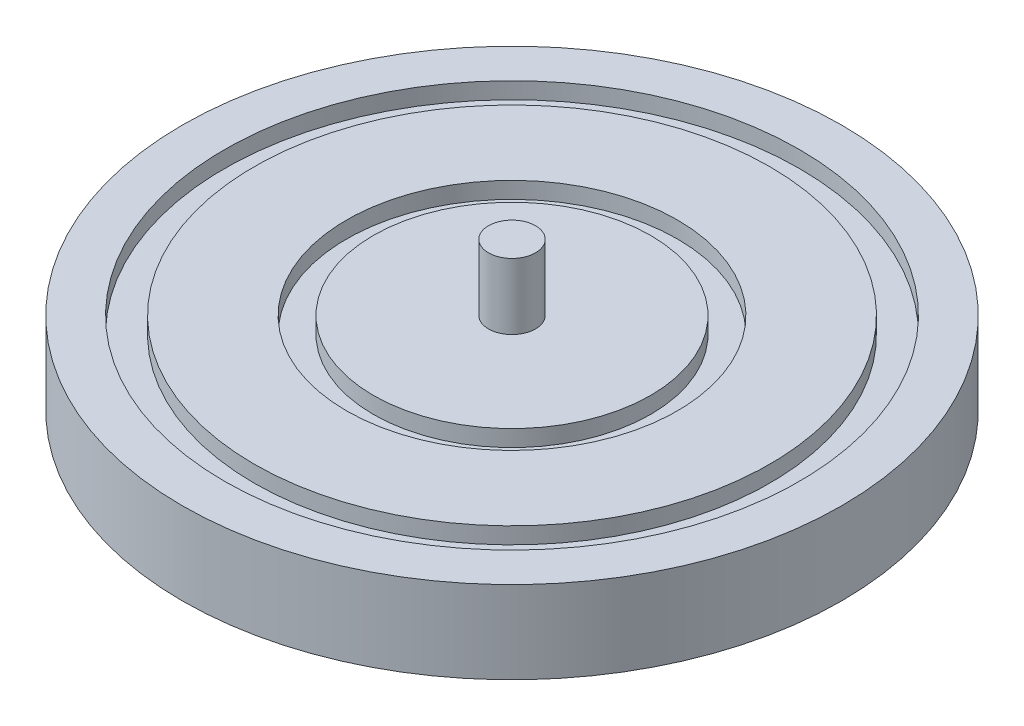
from build123d import *

# Parameters (mm, degrees)
SKETCH_1_R          = 20
EXTRUDE_1_DEPTH     = 5
SKETCH_2_R          = 5
EXTRUDE_2_DEPTH     = 6
SKETCH_3_R          = 11.669468733
SKETCH_3_R_2        = 9.545408708
CUT_EXTRUDE_1_DEPTH = 1
SKETCH_4_R          = 1.425
EXTRUDE_3_DEPTH     = 4
SKETCH_5_R          = 17.435273898
SKETCH_5_R_2        = 15.634190673
CUT_EXTRUDE_2_DEPTH = 1
SKETCH_6_R          = 10.034081131
SKETCH_6_R_2        = 8.408881881
CUT_EXTRUDE_3_DEPTH = 1


with BuildPart() as part:
    # 草图1 → 凸台-拉伸1 (new body)
    with BuildSketch(Plane(origin=(0, 0, 0), x_dir=(1, 0, 0), z_dir=(0, 1, 0))):
        with Locations(Location((0, 0, 0), (0, 0, 270))):
            Circle(SKETCH_1_R)
    extrude(amount=EXTRUDE_1_DEPTH)

    # 草图2 → 凸台-拉伸2 (add)
    with BuildSketch(Plane.XZ):
        with Locations(Location((0, 0, 0), (0, 0, 270))):
            Circle(SKETCH_2_R)
    extrude(amount=EXTRUDE_2_DEPTH)

    # 草图3 → 切除-拉伸1 (cut)
    with BuildSketch(Plane.XZ):
        with Locations(Location((0, 0, 0), (0, 0, 270))):
            Circle(SKETCH_3_R)
        with Locations(Location((0, 0, 0), (0, 0, 270))):
            Circle(SKETCH_3_R_2, mode=Mode.SUBTRACT)
    extrude(amount=-CUT_EXTRUDE_1_DEPTH, mode=Mode.SUBTRACT)

    # 草图4 → 凸台-拉伸3 (add)
    with BuildSketch(Plane(origin=(0, 5, 0), x_dir=(1, 0, 0), z_dir=(0, 1, 0))):
        with Locations(Location((0, 0, 0), (0, 0, 270))):
            Circle(SKETCH_4_R)
    extrude(amount=EXTRUDE_3_DEPTH)

    # 草图5 → 切除-拉伸2 (cut)
    with BuildSketch(Plane(origin=(0, 5, 0), x_dir=(1, 0, 0), z_dir=(0, 1, 0))):
        with Locations(Location((0, 0, 0), (0, 0, 270))):
            Circle(SKETCH_5_R)
        with Locations(Location((0, 0, 0), (0, 0, 270))):
            Circle(SKETCH_5_R_2, mode=Mode.SUBTRACT)
    extrude(amount=-CUT_EXTRUDE_2_DEPTH, mode=Mode.SUBTRACT)

    # 草图6 → 切除-拉伸3 (cut)
    with BuildSketch(Plane(origin=(0, 5, 0), x_dir=(1, 0, 0), z_dir=(0, 1, 0))):
        with Locations(Location((0, 0, 0), (0, 0, 270))):
            Circle(SKETCH_6_R)
        with Locations(Location((0, 0, 0), (0, 0, 270))):
            Circle(SKETCH_6_R_2, mode=Mode.SUBTRACT)
    extrude(amount=-CUT_EXTRUDE_3_DEPTH, mode=Mode.SUBTRACT)


solid = part.part
